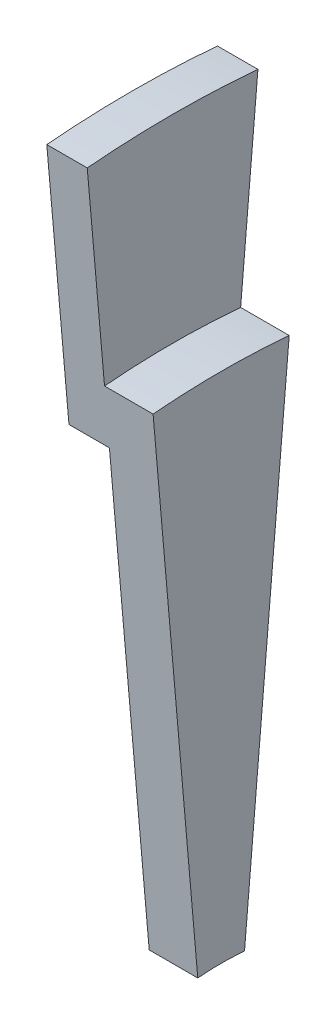
from build123d import *

# Parameters (mm, degrees)
REVOLVE1_ANGLE = 10


with BuildPart() as part:
    # Sketch1 → Revolve1 (revolve, symmetric)
    with BuildSketch(Plane.XY) as revolve1_sk:
        Polygon((-109.954236571, 39.405686592), (-109.954236571, 31.426003585), (-108, 31.426003585), (-108, 10.794907178), (-109.954236571, 10.794907178), (-109.954236571, 29.163164129), (-111.581862319, 29.163164129), (-111.581862319, 39.405686592), align=None)
    revolve(axis=Axis((0, 0, 0), (-1, 0, 0)), revolution_arc=REVOLVE1_ANGLE / 2)
    revolve(revolve1_sk.sketch, axis=Axis((0, 0, 0), (1, 0, 0)), revolution_arc=REVOLVE1_ANGLE / 2)


solid = part.part
